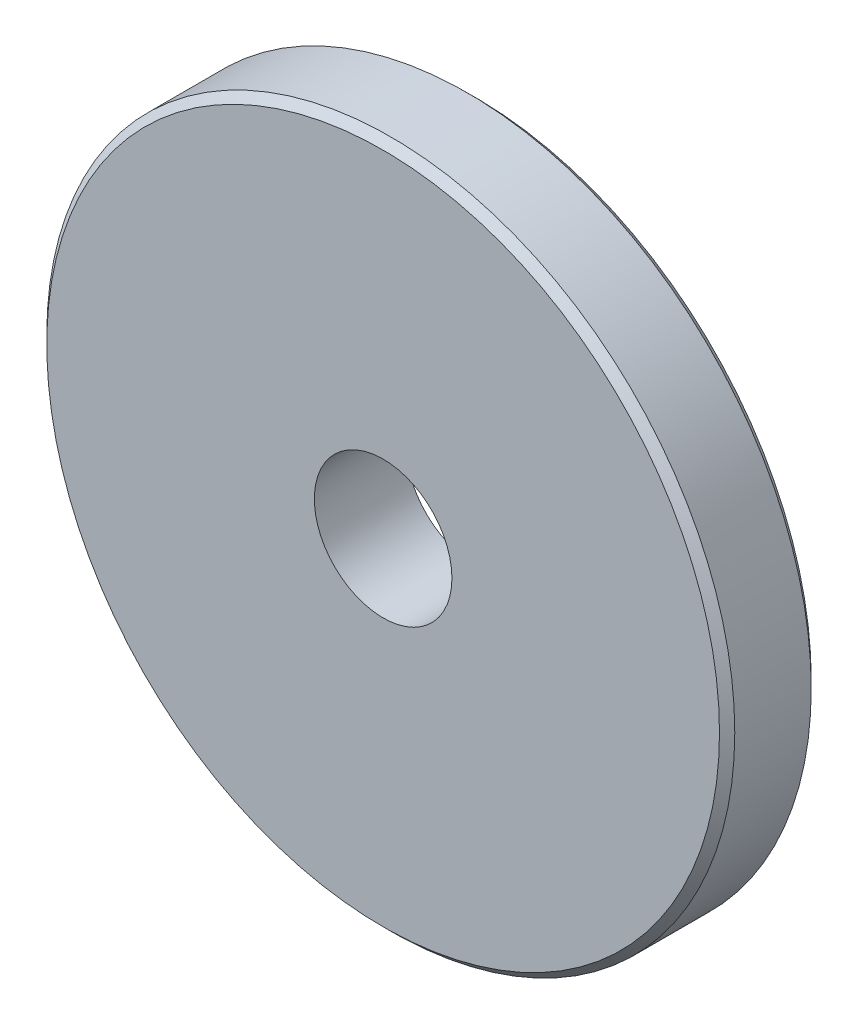
from build123d import *

# Parameters (mm, degrees)
SKETCH_1_R      = 22.5
SKETCH_1_R_2    = 4.5
EXTRUDE_1_DEPTH = 6
CHAMFER_1_SIZE  = 0.5


with BuildPart() as part:
    # 草图1 → 凸台-拉伸1 (new body)
    with BuildSketch(Plane.XY):
        Circle(SKETCH_1_R)
        Circle(SKETCH_1_R_2, mode=Mode.SUBTRACT)
    extrude(amount=EXTRUDE_1_DEPTH)

    # 倒角1
    chamfer_1_edges = [part.edges().sort_by_distance(p)[0] for p in [
        (-22.5, 0, 0),
        (-22.5, 0, 6),
    ]]
    chamfer(chamfer_1_edges, length=CHAMFER_1_SIZE)


solid = part.part
